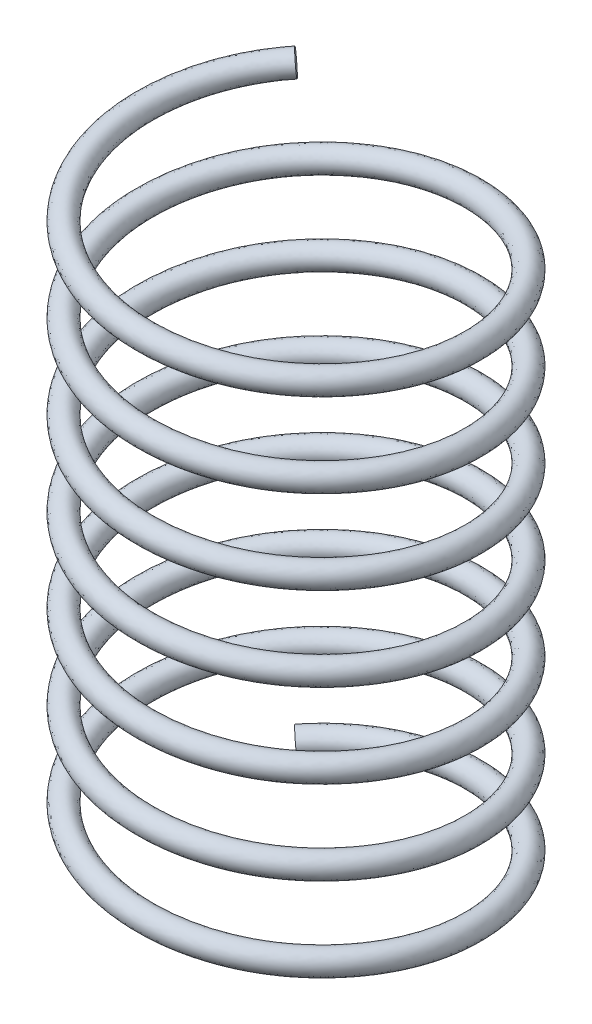
from build123d import *

# Parameters (mm, degrees)
SWEEP1_PITCH       = 1.428571429
SWEEP1_HEIGHT      = 10
SWEEP1_RADIUS      = 2.8
SWEEP1_START_ANGLE = -135
SKETCH2_R          = 0.2


with BuildPart() as part:
    # Sweep1: sweep along a helix
    with BuildLine() as sweep1_path:
        add(Helix(SWEEP1_PITCH, SWEEP1_HEIGHT, SWEEP1_RADIUS, center=(0, 0, 0), direction=(0, 1, 0), lefthand=True, mode=Mode.PRIVATE).rotate(Axis((0, 0, 0), (0, 1, 0)), SWEEP1_START_ANGLE))
    # Sketch2 → Sweep1 (sweep)
    with BuildSketch(Plane(origin=(-1.979898987, 10, -1.979898987), x_dir=(0.7001385575920928, 0.08081360418948051, 0.709418890043654), z_dir=(0.7047870274114748, 0.08093510971866495, -0.7047870274113484))):
        Circle(SKETCH2_R)
    sweep(path=sweep1_path.line, is_frenet=True)


solid = part.part
